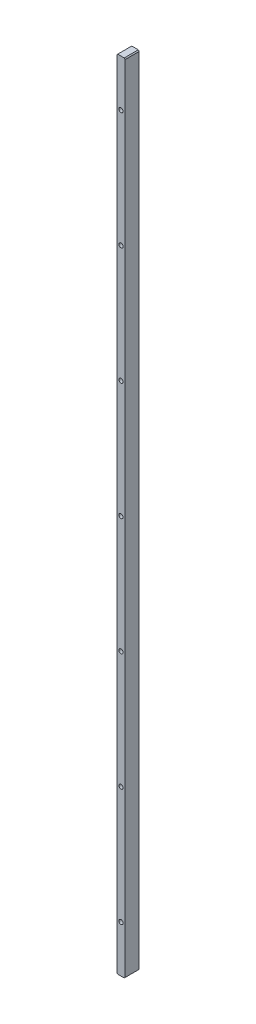
from build123d import *

# Parameters (mm, degrees)
SKETCH_1_W                   = 18
SKETCH_1_H                   = 30
EXTRUDE_1_DEPTH              = 1700
CHAMFER_1_SIZE               = 2
HOLE_WIZARD_M8_1_D           = 9
HOLE_WIZARD_M8_1_CBORE_D     = 15
HOLE_WIZARD_M8_1_CBORE_DEPTH = 19


with BuildPart() as part:
    # 草图1 → 凸台-拉伸1 (new body)
    with BuildSketch(Plane(origin=(0, 0, 0), x_dir=(1, 0, 0), z_dir=(0, 1, 0))):
        with Locations((9, 15)):
            Rectangle(SKETCH_1_W, SKETCH_1_H)
    extrude(amount=EXTRUDE_1_DEPTH)

    # 倒角1
    chamfer_1_edges = [part.edges().sort_by_distance(p)[0] for p in [
        (18, 1700, -15),
        (0, 1700, -15),
        (18, 0, -15),
        (0, 0, -15),
    ]]
    chamfer(chamfer_1_edges, length=CHAMFER_1_SIZE)

    # M8 六角圆柱头螺钉的柱形沉头孔1 (through all)
    with Locations(Plane(origin=(0, 0, -30), x_dir=(-1, 0, 0), z_dir=(0, 0, -1))):
        with Locations((-9, 1600), (-9, 1350), (-9, 1100), (-9, 600), (-9, 350), (-9, 100), (-9, 850)):
            CounterBoreHole(HOLE_WIZARD_M8_1_D / 2, HOLE_WIZARD_M8_1_CBORE_D / 2, HOLE_WIZARD_M8_1_CBORE_DEPTH)


solid = part.part
